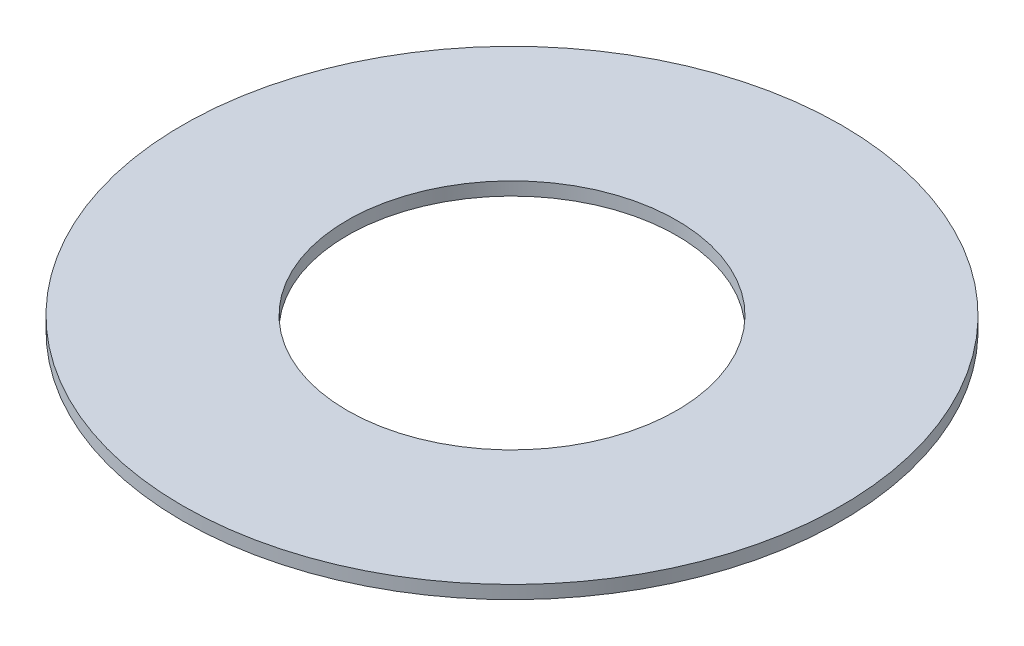
SolidWorks part; units mm, degrees
material "HT200"
ref_plane "Front Plane" through (0, 0, 0) normal (0, 0, 1) x (1, 0, 0)
ref_plane "Top Plane" through (0, 0, 0) normal (0, 1, 0) x (1, 0, 0)
ref_plane "Right Plane" through (0, 0, 0) normal (1, 0, 0) x (0, 0, -1)
other "Configuration Table"
sketch "Sketch1" plane through (0, 0, 0) normal (0, 1, 0) x (1, 0, 0)
  circle A0 centre (0, 0) radius 50
  circle A1 centre (0, 0) radius 25
  dimension "D1" = 100
  dimension "D2" = 50
extrude "Boss-Extrude1" add sketch "Sketch1" along normal blind 2
